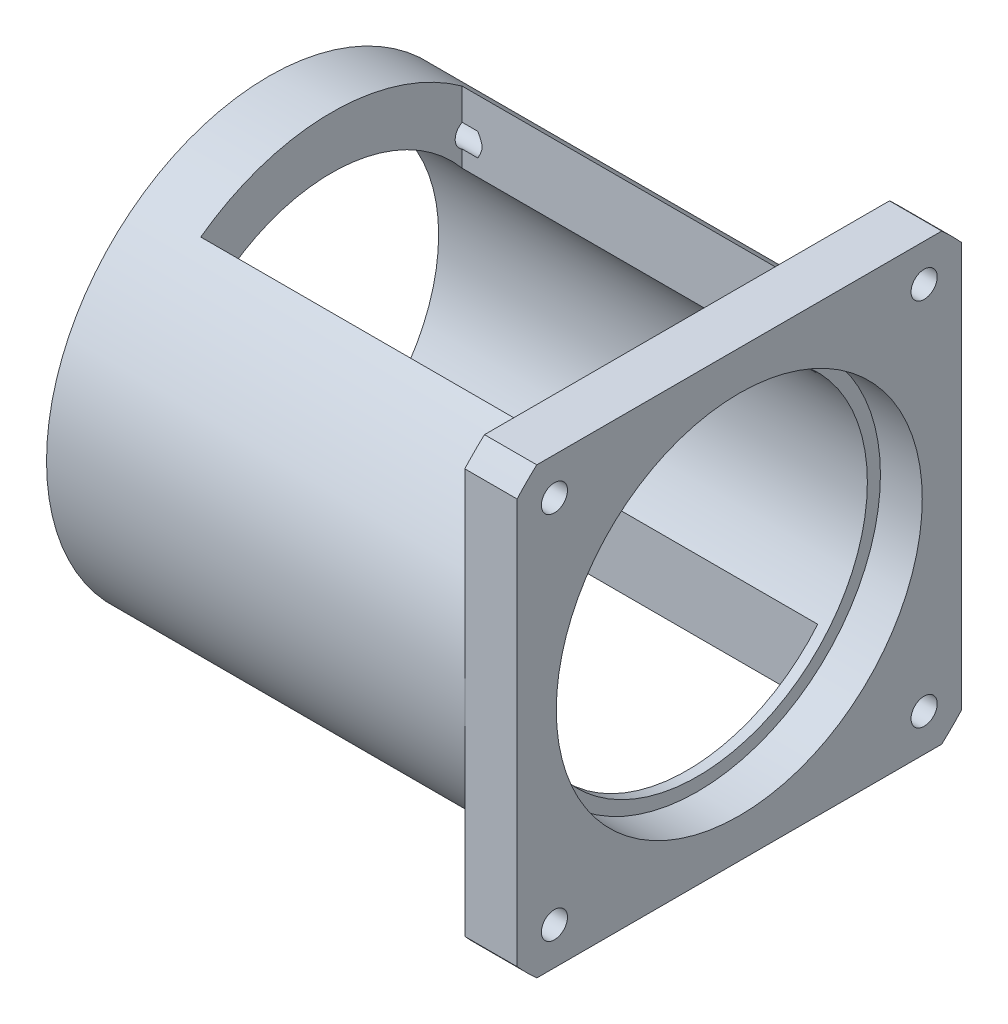
SolidWorks part; units mm, degrees
ref_plane "前视基准面" through (0, 0, 0) normal (0, 0, 1) x (1, 0, 0)
ref_plane "上视基准面" through (0, 0, 0) normal (0, 1, 0) x (1, 0, 0)
ref_plane "右视基准面" through (0, 0, 0) normal (1, 0, 0) x (0, 0, -1)
sketch "草图1" plane through (0, 0, 0) normal (1, 0, 0) x (0, 0, -1)
  circle A0 centre (0, 0) radius 42.5
  dimension "D1" = 85
extrude "凸台-拉伸1" add sketch "草图1" along normal blind 80
sketch "草图2" plane through (80, 0, 0) normal (1, 0, 0) x (0, 0, -1)
  circle A0 centre (0, 0) radius 57.5
  dimension "D1" = 115
extrude "凸台-拉伸2" add sketch "草图2" along normal blind 10
sketch "草图3" plane through (90, 0, 0) normal (1, 0, 0) x (0, 0, -1)
  line L0 (0, 132.3949) -> (0, 0) construction
  line L1 (-42.5, 42.5) -> (42.5, 42.5)
  line L2 (-42.5, 42.5) -> (-42.5, -42.5)
  line L3 (-42.5, -42.5) -> (42.5, -42.5)
  line L4 (42.5, 42.5) -> (42.5, -42.5)
  line L5 (0, 0) -> (118.7422, 0) construction
  dimension "D1" = 85
extrude "切除-拉伸1" cut sketch "草图3" against normal through all flip side to cut
sketch "草图4" plane through (90, 0, 0) normal (1, 0, 0) x (0, 0, -1)
  circle A0 centre (0, 0) radius 35
  dimension "D1" = 70
extrude "切除-拉伸2" cut sketch "草图4" against normal blind 8
hole_wizard "M6 螺纹孔1" positions "草图5" profile "草图6" tap size "M6" standard "GB"
sketch "草图5" plane through (90, 0, 0) normal (1, 0, 0) x (0, 0, -1)
  line L0 (0, 0) -> (0, 62.713) construction
  line L2 (0, 0) -> (-35.3553, 35.3553) construction
  point P0 (-35.3553, 35.3553)
  dimension "D1" = 45
  dimension "D2" = 50
sketch "草图6" plane through (90, 35.3553, 35.3553) normal (0, 1, 0) x (0, 0, -1)
  line L0 (0, 0) -> (0, 16.5022)
  line L1 (0, 16.5022) -> (2.5, 15)
  line L2 (2.5, 15) -> (2.5, 0)
  line L5 (2.5, 0) -> (0, 0)
  line L10 (0, 16.5022) -> (-2.5, 15) construction
  line L11 (0, -6.35) -> (0, 107.95) construction
  dimension "螺纹孔钻头直径" = 5
  dimension "螺纹孔钻头深度" = 15
  dimension "导头角度" = 118
cosmetic thread "孔螺蚊线1" parameters "D1"=10, "D2"=6
pattern_circular "阵列(圆周)1" count 4 over 360 about axis through (0, 0, 0) along (1, 0, 0) of "M6 螺纹孔1"
sketch "草图7" plane through (82, 0, 0) normal (1, 0, 0) x (0, 0, -1)
  circle A0 centre (0, 0) radius 32.5
  dimension "D1" = 65
extrude "切除-拉伸3" cut sketch "草图7" against normal through all
sketch "草图8" plane through (0, 0, 0) normal (0, 1, 0) x (1, 0, 0)
  line L0 (0, 0) -> (80.8943, 0) construction
  line L1 (12, 25) -> (80, 25)
  line L2 (12, 25) -> (12, -25)
  line L3 (12, -25) -> (80, -25)
  line L4 (80, 25) -> (80, -25)
  line L5 (80, 38.7298) -> (80, 0) construction
  line L6 (0, 42.5) -> (0, -42.5) construction
  dimension "D1" = 50
  dimension "D2" = 12
extrude "切除-拉伸4" cut sketch "草图8" against normal through all both and the other way through all
hole_wizard "M6 螺纹孔2" positions "草图9" profile "草图10" tap size "M6" standard "GB"
sketch "草图9" plane through (0, 0, 0) normal (-1, 0, 0) x (0, 0, 1)
  line L0 (0, 0) -> (-26.163, 26.163) construction
  line L2 (0, 0) -> (0, 25.4931) construction
  point P0 (-26.163, 26.163)
  dimension "D1" = 45
  dimension "D2" = 37
sketch "草图10" plane through (0, 26.163, -26.163) normal (0, 1, 0) x (0, 0, 1)
  line L0 (0, 0) -> (0, 16.5022)
  line L1 (0, 16.5022) -> (2.5, 15)
  line L2 (2.5, 15) -> (2.5, 0)
  line L5 (2.5, 0) -> (0, 0)
  line L10 (0, 16.5022) -> (-2.5, 15) construction
  line L11 (0, -6.35) -> (0, 107.95) construction
  dimension "螺纹孔钻头直径" = 5
  dimension "螺纹孔钻头深度" = 15
  dimension "导头角度" = 118
cosmetic thread "孔螺蚊线2" parameters "D1"=12, "D2"=6
pattern_circular "阵列(圆周)2" count 4 over 360 about axis through (0, 0, 0) along (1, 0, 0) of "M6 螺纹孔2"
